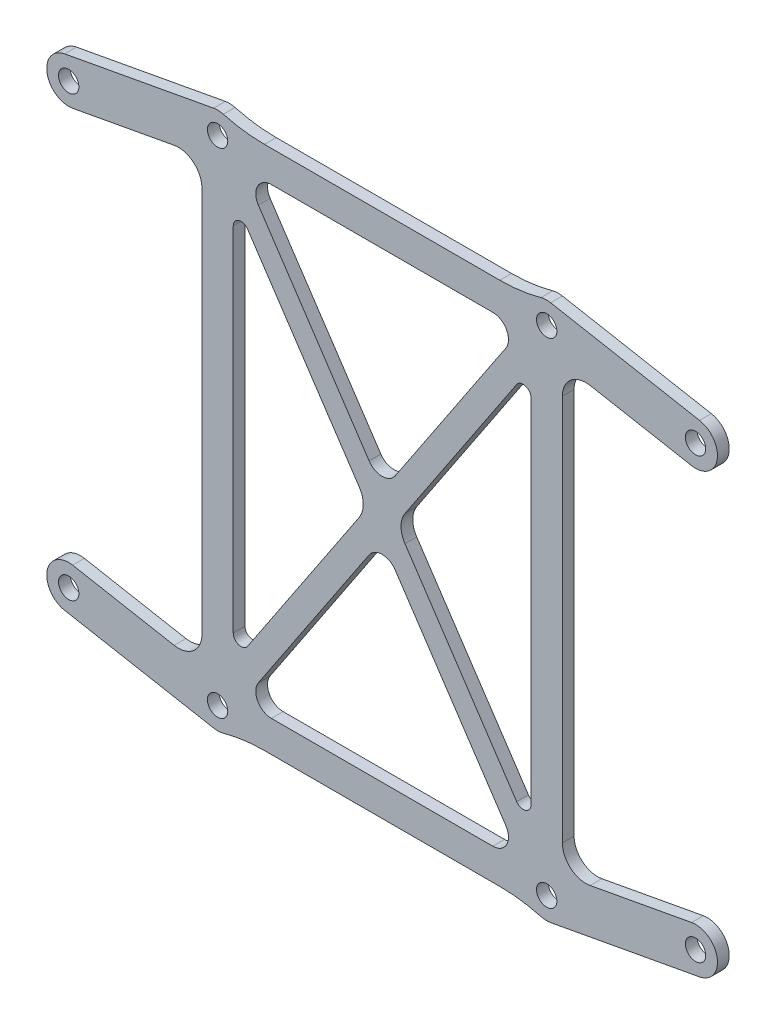
from build123d import *

# Parameters (mm, degrees)
SKETCH_1_R      = 1.3
EXTRUDE_1_DEPTH = 1.5
FILLET_1_R      = 2
FILLET_2_R      = 1
FILLET_3_R      = 20
FILLET_4_R      = 3


with BuildPart() as part:
    # 草图1 → 凸台-拉伸1 (new body)
    with BuildSketch(Plane.XY):
        with BuildLine():
            Line((-19.040408206, -33.5), (19.040408206, -33.5))
            ThreePointArc((19.040408206, -33.5), (20.181877211, -34.177811626), (21.507254803, -34.253668928))
            Line((21.507254803, -34.253668928), (40.507254803, -30.753668928))
            ThreePointArc((40.507254803, -30.753668928), (42.753668928, -27.492745197), (39.492745197, -25.246331072))
            Line((39.492745197, -25.246331072), (23, -28.284468345))
            Line((23, -28.284468345), (23, 28.284468345))
            Line((23, 28.284468345), (39.492745197, 25.246331072))
            ThreePointArc((39.492745197, 25.246331072), (42.753668928, 27.492745197), (40.507254803, 30.753668928))
            Line((40.507254803, 30.753668928), (21.507254803, 34.253668928))
            ThreePointArc((21.507254803, 34.253668928), (20.181877211, 34.177811626), (19.040408206, 33.5))
            Line((19.040408206, 33.5), (-19.040408206, 33.5))
            ThreePointArc((-19.040408206, 33.5), (-20.181877211, 34.177811626), (-21.507254803, 34.253668928))
            Line((-21.507254803, 34.253668928), (-40.507254803, 30.753668928))
            ThreePointArc((-40.507254803, 30.753668928), (-42.753668928, 27.492745197), (-39.492745197, 25.246331072))
            Line((-39.492745197, 25.246331072), (-23, 28.284468345))
            Line((-23, 28.284468345), (-23, -28.284468345))
            Line((-23, -28.284468345), (-39.492745197, -25.246331072))
            ThreePointArc((-39.492745197, -25.246331072), (-42.753668928, -27.492745197), (-40.507254803, -30.753668928))
            Line((-40.507254803, -30.753668928), (-21.507254803, -34.253668928))
            ThreePointArc((-21.507254803, -34.253668928), (-20.181877211, -34.177811626), (-19.040408206, -33.5))
        make_face()
        with Locations((-40, -28)):
            Circle(SKETCH_1_R, mode=Mode.SUBTRACT)
        with Locations((-21, -31.5)):
            Circle(SKETCH_1_R, mode=Mode.SUBTRACT)
        with Locations((40, -28)):
            Circle(SKETCH_1_R, mode=Mode.SUBTRACT)
        Polygon((0, -2.704163457), (17.863891029, -29.5), (-17.863891029, -29.5), align=None, mode=Mode.SUBTRACT)
        Polygon((-19, 25.795836543), (-1.802775638, 0), (-19, -25.795836543), align=None, mode=Mode.SUBTRACT)
        with Locations((-40, 28)):
            Circle(SKETCH_1_R, mode=Mode.SUBTRACT)
        with Locations((-21, 31.5)):
            Circle(SKETCH_1_R, mode=Mode.SUBTRACT)
        Polygon((19, -25.795836543), (1.802775638, 0), (19, 25.795836543), align=None, mode=Mode.SUBTRACT)
        Polygon((0, 2.704163457), (-17.863891029, 29.5), (17.863891029, 29.5), align=None, mode=Mode.SUBTRACT)
        with Locations((21, 31.5)):
            Circle(SKETCH_1_R, mode=Mode.SUBTRACT)
        with Locations((40, 28)):
            Circle(SKETCH_1_R, mode=Mode.SUBTRACT)
        with Locations((21, -31.5)):
            Circle(SKETCH_1_R, mode=Mode.SUBTRACT)
    extrude(amount=EXTRUDE_1_DEPTH)

    # 圆角1
    fillet_1_edges = [part.edges().sort_by_distance(p)[0] for p in [
        (17.863891029, -29.5, 0.75),
        (0, -2.704163457, 0.75),
        (-17.863891029, -29.5, 0.75),
        (-17.863891029, 29.5, 0.75),
        (0, 2.704163457, 0.75),
        (17.863891029, 29.5, 0.75),
    ]]
    fillet(fillet_1_edges, radius=FILLET_1_R)

    # 圆角2
    fillet_2_edges = [part.edges().sort_by_distance(p)[0] for p in [
        (19, -25.795836543, 0.75),
        (19, 25.795836543, 0.75),
        (-19, 25.795836543, 0.75),
        (-19, -25.795836543, 0.75),
    ]]
    fillet(fillet_2_edges, radius=FILLET_2_R)

    # 圆角3
    fillet_3_edges = [part.edges().sort_by_distance(p)[0] for p in [
        (19.040408206, 33.5, 0.75),
        (19.040408206, -33.5, 0.75),
        (-19.040408206, -33.5, 0.75),
        (-19.040408206, 33.5, 0.75),
    ]]
    fillet(fillet_3_edges, radius=FILLET_3_R)

    # 圆角4
    fillet_4_edges = [part.edges().sort_by_distance(p)[0] for p in [
        (1.802775638, 0, 0.75),
        (-1.802775638, 0, 0.75),
        (23, 28.284468345, 0.75),
        (23, -28.284468345, 0.75),
        (-23, -28.284468345, 0.75),
        (-23, 28.284468345, 0.75),
    ]]
    fillet(fillet_4_edges, radius=FILLET_4_R)


solid = part.part
